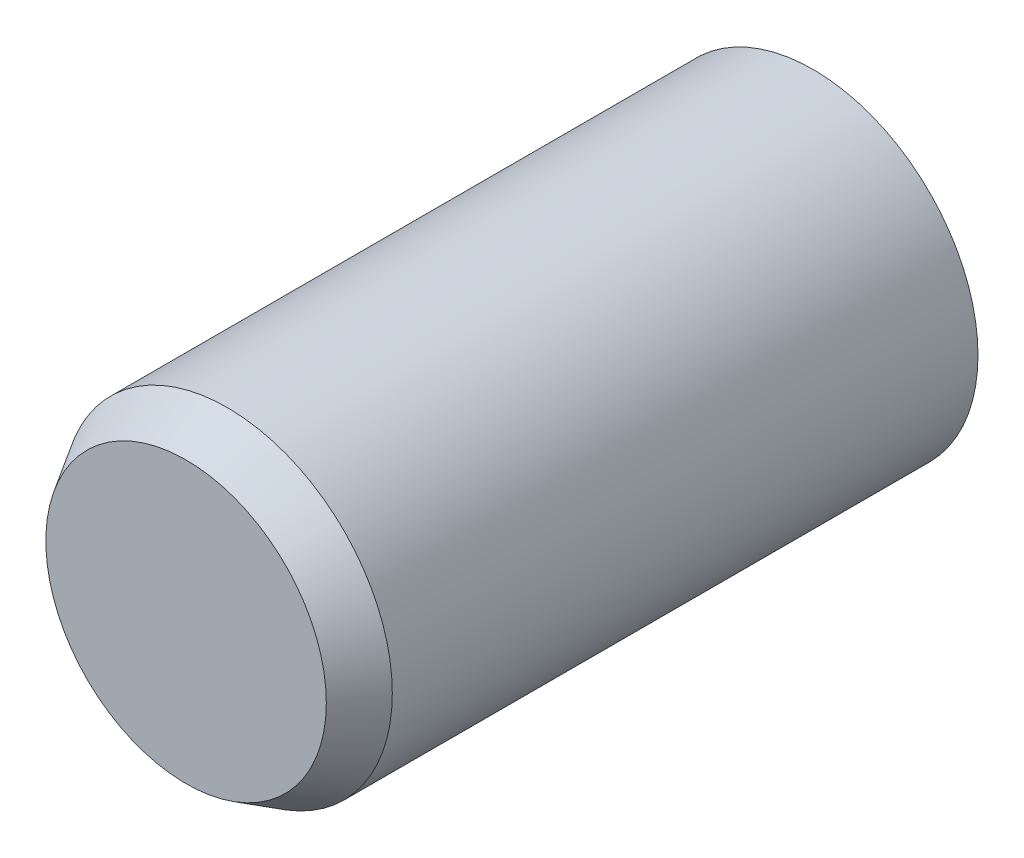
from build123d import *

# Parameters (mm, degrees)
SKETCH1_R             = 40
BOSS_EXTRUDE1_DEPTH   = 152
CHAMFER1_SIZE         = 10
CHAMFER1_SIZE2        = 6
M6_TAPPED_HOLE1_D     = 5
M6_TAPPED_HOLE1_DEPTH = 17
M6_TAPPED_HOLE1_TIP   = 1.502151548


with BuildPart() as part:
    # Sketch1 → Boss-Extrude1 (new body)
    with BuildSketch(Plane.XY):
        Circle(SKETCH1_R)
    extrude(amount=BOSS_EXTRUDE1_DEPTH)

    # Chamfer1
    chamfer1_edges = [part.edges().sort_by_distance(p)[0] for p in [
        (-40, 0, 152),
    ]]
    chamfer1_side = [part.faces().sort_by_distance(p)[0] for p in [
        (-40, 0, 76),
    ]]
    chamfer(chamfer1_edges, length=CHAMFER1_SIZE, length2=CHAMFER1_SIZE2, reference=chamfer1_side[0])

    # M6 Tapped Hole1
    with Locations(Plane(origin=(0, 0, 0), x_dir=(-1, 0, 0), z_dir=(0, 0, -1))):
        with Locations((0, 0)):
            Hole(M6_TAPPED_HOLE1_D / 2, depth=M6_TAPPED_HOLE1_DEPTH)
            with Locations((0, 0, -(M6_TAPPED_HOLE1_DEPTH + M6_TAPPED_HOLE1_TIP / 2))):  # 118° drill point
                Cone(0, M6_TAPPED_HOLE1_D / 2, M6_TAPPED_HOLE1_TIP, mode=Mode.SUBTRACT)


solid = part.part
